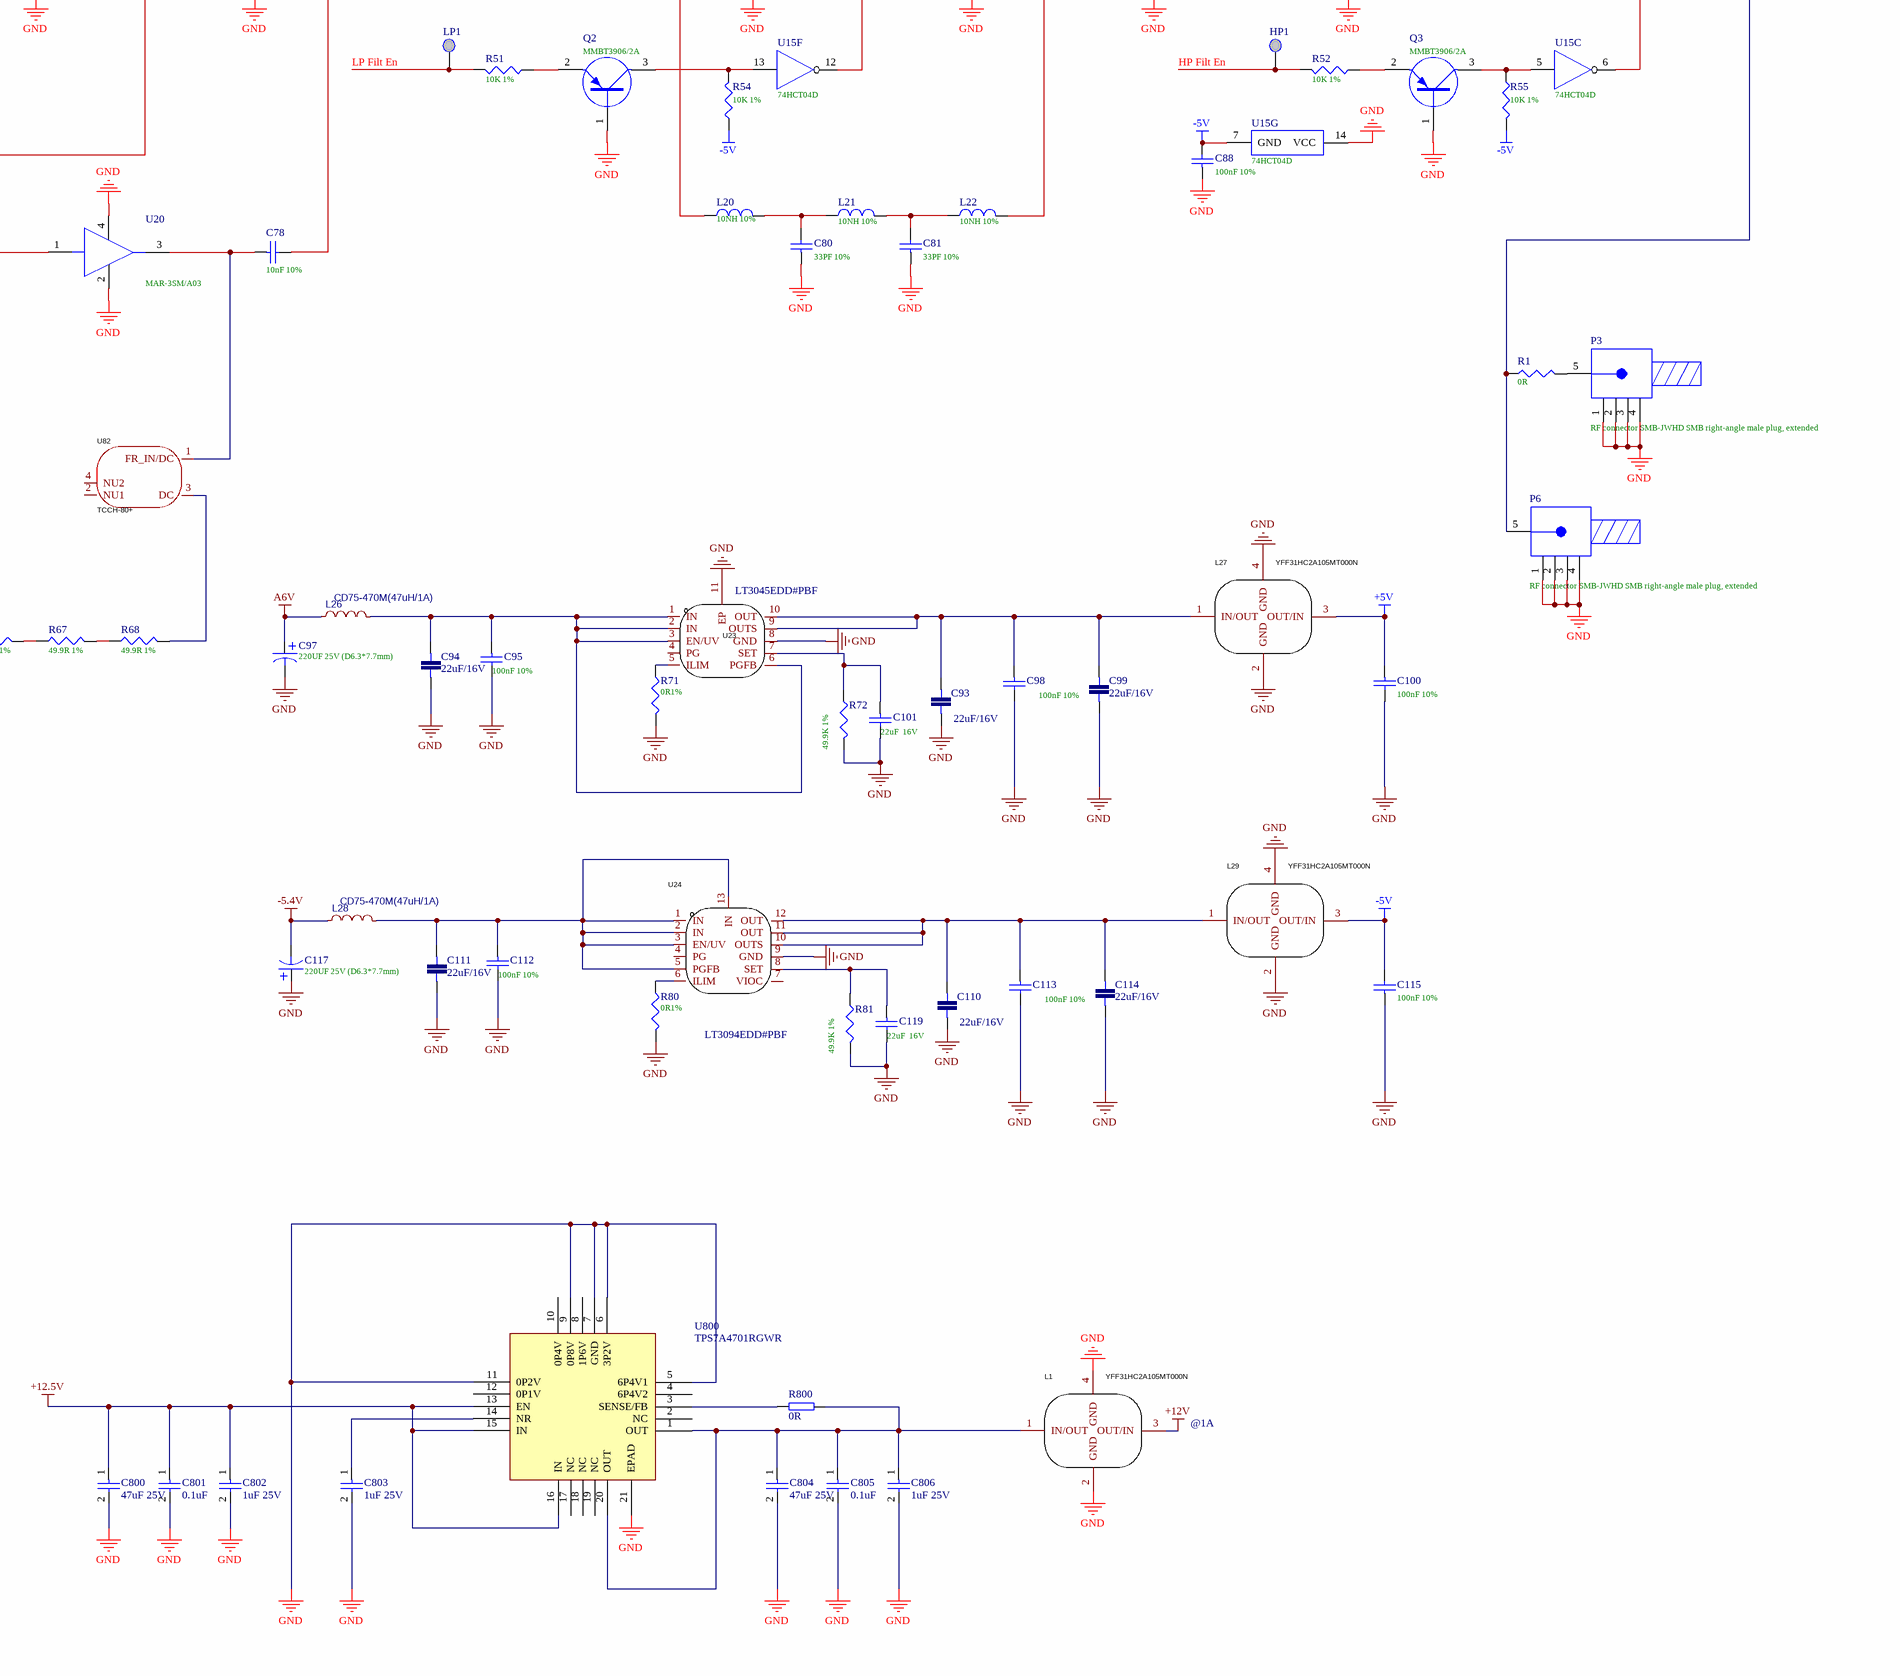
[diagram p0: PCBE109560-12.SchDoc, bottom right]
# Altium project MISC109560-2.PrjPcb (part 2 of 2)

## Sheet PCBE109560-12.SchDoc
size E; SheetNumber: 0; SheetTotal: 0

### Parts
1  (no value)  [DIP-1]
+1  (no value)  [DIP-1]
+2  (no value)  [DIP-1]
C4  20PF 10%  [0805C-2]
C5  330PF 10%  [1812C]
C6  22PF 10%  [1812C-2]
C7  22uF/16V  [0805]
C8  22uF/16V  [0805]
C9  100nF 10%  [0603]
C10  220UF 25V (D6.3*7.7mm)  [CAP-SMD_BD6.3-L6.6-W6.6-FD]
C11  100nF 10%  [0603]
C12  22uF/16V  [0805]
C13  100nF 10%  [0805R]
C14  22uF  16V  [0805]
C15  100nF 10%  [0805R]
C16  47PF 10%  [1812C-2]
C17  100PF 10%  [1812C-2]
C18  20PF 10%  [0805R]
C20  100nF 10%  [0805R]
C21  100nF 10%  [0805R]
C31  100nF 10%  [0805R]
C32  100nF 10%  [0805R]
C34  100nF 10%  [0805R]
C35  100nF 10%  [0805R]
C36  100nF 10%  [0805R]
C37  100nF 10%  [0805R]
C39  100nF 10%  [0805R]
C40  100nF 10%  [0805R]
C41  100nF 10%  [0805R]
C42  100nF 10%  [0805R]
C43  100nF 10%  [0805R]
C44  100nF 10%  [0805R]
C45  100nF 10%  [0805R]
C46  100nF 10%  [0805R]
C47  100nF 10%  [0805R]
C48  100nF 10%  [0805R]
C49  22uF 25V  [CAP-SMD_L6.0-W3.2-R-RD]
C50  100nF 10%  [0805R]
C51  100nF 10%  [0805R]
C52  100nF 10%  [0805R]
C53  3.3NF 10%  [0805R]
C54  100nF 10%  [0805R]
C55  330PF 10%  [0805R]
C56  330PF 10%  [0805R]
C57  100nF 10%  [0805R]
C58  33PF 10%  [0805R]
C59  33PF 10%  [0805R]
C60  100nF 10%  [0805R]
C61  100nF 10%  [0805R]
C62  100nF 10%  [0805R]
C63  100nF 10%  [0805R]
C64  100nF 10%  [0805R]
C65  33PF 10%  [0805R]
C66  33PF 10%  [0805R]
C67  100nF 10%  [0805R]
C68  39PF 10%  [0805R]
C69  100nF 10%  [0805R]
C70  25V 1UF Type A  [0805C-2]
C71  25V 1UF Type A  [0805C-2]
C72  100nF 10%  [0805R]
C73  25V 1UF Type A  [0805C-2]
C74  100nF 10%  [0805R]
C75  100nF 10%  [0805R]
C76  10nF 10%  [0805R]
C77  10nF 10%  [0805R]
C78  10nF 10%  [0805R]
C79  100nF 10%  [0603C]
C80  33PF 10%  [0805R]
C81  33PF 10%  [0805R]
C82  100nF 10%  [0805R]
C83  100nF 10%  [0805R]
C84  100nF 10%  [0805R]
C85  100nF 10%  [0805R]
C86  25V 1UF Type A  [0805C-2]
C87  3pF( ±0.1pF)  [0805R]
C88  100nF 10%  [0805R]
C89  100nF 10%  [0805R]
C90  100nF 10%  [0805R]
C93  22uF/16V  [0805]
C94  22uF/16V  [0805]
C95  100nF 10%  [0603]
C96  100nF 10%  [0805R]
C97  220UF 25V (D6.3*7.7mm)  [CAP-SMD_BD6.3-L6.6-W6.6-FD]
C98  100nF 10%  [0603]
C99  22uF/16V  [0805]
C100  100nF 10%  [0805R]
C101  22uF  16V  [0805]
C102  100nF 10%  [0805R]
C103  100nF 10%  [0805R]
C104  100nF 10%  [0805R]
C105  100nF 10%  [0805R]
C106  100nF 10%  [0805R]
C107  100nF 10%  [0805R]
C109  100nF 10%  [0805R]
C110  22uF/16V  [0805]
C111  22uF/16V  [0805]
C112  100nF 10%  [0603]
C113  100nF 10%  [0603]
C114  22uF/16V  [0805]
C115  100nF 10%  [0805R]
C116  100nF 10%  [0805R]
C117  220UF 25V (D6.3*7.7mm)  [CAP-SMD_BD6.3-L6.6-W6.6-FD]
C118  100nF 10%  [0805R]
C119  22uF  16V  [0805]
C122  100nF 10%  [0805R]
C123  100nF 10%  [0805R]
C124  100nF 10%  [0805R]
C125  100nF 10%  [0805R]
C128  100nF 10%  [0805R]
C129  100nF 10%  [0805R]
C130  100nF 10%  [0805R]
C800  47uF 25V  [1206]
C801  0.1uF  [0402]
C802  1uF 25V  [0402]
C803  1uF 25V  [0402]
C804  47uF 25V  [1206]
C805  0.1uF  [0402]
C806  1uF 25V  [0402]
C809  100nF 10%  [0805R]
C888  100nF 10%  [0805R]
Clk1  (no value)  [DIP-1]
D1  BAV99/A7  [SOT-23]
D2  GF1M-E3/67A/GM  [1808D]
D3  GF1M-E3/67A/GM  [1808D]
D4  GF1M-E3/67A/GM  [1808D]
D5  GF1M-E3/67A/GM  [1808D]
D8  BAV99/A7  [SOT-23-2]
D9  BAV99/A7  [SOT-23-2]
D10  BAV99/A7  [SOT-23-2]
D11  BAV99/A7  [SOT-23-2]
D12  BAV99/A7  [SOT-23-2]
Data1  (no value)  [DIP-1]
HP1  (no value)  [DIP-1]
J1  RF connector  [DIP-P]
J2  RF connector  [DIP-P]
L1  YFF31HC2A105MT000N  [FILTER-SMD_4P-L3.2-W1.6-L_YFF31HC]
L2  15UH 5%  [1005R]
L3  BLM21PG221SN1D(220Ω@100MHz)  [0805R]
L4  YFF31HC2A105MT000N  [FILTER-SMD_4P-L3.2-W1.6-L_YFF31HC]
L5  6.8UH 10%  [0805R]
L8  YFF31HC2A105MT000N  [FILTER-SMD_4P-L3.2-W1.6-L_YFF31HC]
L10  10NH 10%  [0805R]
L11  10NH 10%  [0805R]
L12  10NH 10%  [0805R]
L13  YFF31HC2A105MT000N  [FILTER-SMD_4P-L3.2-W1.6-L_YFF31HC]
L15  4.7UH 5%  [1005L]
L16  1UH 5%  [0805R]
L17  BLM21PG221SN1D(220Ω@100MHz)  [0805R]
L18  BLM21PG221SN1D(220Ω@100MHz  [0805R]
L19  NFM15PC104R1A3D  [FILTER-SMD_0402-3P-L1.0-W0.5-T]
L20  10NH 10%  [0805R]
L21  10NH 10%  [0805R]
L22  10NH 10%  [0805R]
L23  YFF31HC2A105MT000N  [FILTER-SMD_4P-L3.2-W1.6-L_YFF31HC]
L24  YFF31HC2A105MT000N  [FILTER-SMD_4P-L3.2-W1.6-L_YFF31HC]
L25  BLM21PG221SN1D(220Ω@100MHz  [0805R]
L26  CD75-470M(47uH/1A)  [IND-SMD_L7.8-W7.0-A]
L27  YFF31HC2A105MT000N  [FILTER-SMD_4P-L3.2-W1.6-L_YFF31HC]
L28  CD75-470M(47uH/1A)  [IND-SMD_L7.8-W7.0-A]
L29  YFF31HC2A105MT000N  [FILTER-SMD_4P-L3.2-W1.6-L_YFF31HC]
L31  BLM21PG221SN1D(220Ω@100MHz  [0805R]
L32  BLM21PG221SN1D(220Ω@100MHz  [0805R]
L808  NFM15PC104R1A3D  [FILTER-SMD_0402-3P-L1.0-W0.5-T]
L809  NFM15PC104R1A3D  [FILTER-SMD_0402-3P-L1.0-W0.5-T]
L810  NFM15PC104R1A3D  [FILTER-SMD_0402-3P-L1.0-W0.5-T]
L811  NFM15PC104R1A3D  [FILTER-SMD_0402-3P-L1.0-W0.5-T]
L812  NFM15PC104R1A3D  [FILTER-SMD_0402-3P-L1.0-W0.5-T]
L813  NFM15PC104R1A3D  [FILTER-SMD_0402-3P-L1.0-W0.5-T]
LP1  (no value)  [DIP-1]
P1  Header 20X2  [N0.8mm/40Pin-Plug]
P2  Header 4X2  [N0.8mm/8Pin-SOCKET]
P3  RF connector SMB-JWHD SMB right-angle male plug, extended  [DIP-P-2]
P4  Header 20X2  [N0.8mm/40Pin-Plug]
P5  Header 20X2  [N0.8mm/40Pin-Plug]
P6  RF connector SMB-JWHD SMB right-angle male plug, extended  [DIP-P-2]
Q1  MJD31C  [SOT-252-2]
Q2  MMBT3906/2A  [SOT-23]
Q3  MMBT3906/2A  [SOT-23]
Q4  MMBT3906/2A  [SOT-23]
R1  0R  [0805R]
R6  2K 5%  [0603]
R7  NC  [AXIAL-0.51]
R8  3.9K 5% 1/2W  [AXIAL-0.51]
R9  3.9K 5% 1/2W  [AXIAL-0.51]
R10  3.9K 5% 1/2W  [AXIAL-0.51]
R11  3.9K 5% 1/2W  [AXIAL-0.51]
R13  0R1%  [0603]
R14  49.9K 1%  [0603]
R15  4.99K 1%  [0805R]
R16  2K 1%  [0805R]
R17  49.9R 1% 1/4W  [AXIAL-0.4]
R20  100R 1% 1/4W  [AXIAL-0.4]
R23  100R 1% 1/4W  [AXIAL-0.4]
R27  4.87K 1%  [0805R]
R28  4.87K 1%  [0805R]
R29  4.87K 1%  [0805R]
R30  4.87K 1%  [0805R]
R31  4.87K 1%  [0805R]
R32  10K 1%  [0805R]
R33  100K 1%  [0805R]
R34  100K 1%  [0805R]
R35  49.9R 1%  [0805R]
R36  49.9R 1%  [0805R]
R37  49.9R 1%  [0805R]
R38  49.9R 1%  [0805R]
R39  49.9R 1%  [0805R]
R40  49.9R 1% 1/4W  [R-SMD_L3.5-W1.5]
R41  10K 1%  [0805R]
R42  4.87K 1%  [0805R]
R43  4.87K 1%  [0805R]
R44  4.87K 1%  [0805R]
R45  4.87K 1%  [0805R]
R46  169R 1%  [0805R]
R47  169R 1%  [0805R]
R48  169R 1%  [0805R]
R49  49.9R 1%  [0805R]
R50  49.9R 1%  [0805R]
R51  10K 1%  [0805R]
R52  10K 1%  [0805R]
R53  10K 1%  [0805R]
R54  10K 1%  [0805R]
R55  10K 1%  [0805R]
R56  10K 1%  [0805R]
R57  10K 1%  [0805R]
R58  49.9R 1%  [0805R]
R59  4.99K 1%  [0805R]
R60  49.9R 1%  [R-SMD_L3.5-W1.5]
R61  30R 1%  [R-SMD_L3.5-W1.5]
R62  169R 1%  [0805R]
R63  169R 1%  [0805R]
R64  169R 1%  [0805R]
R65  49.9R 1%  [0805R]
R66  49.9R 1%  [0805R]
R67  49.9R 1%  [0805R]
R68  49.9R 1%  [0805R]
R69  120R 1%  [R-SMD_L3.5-W1.5]
R70  169R 1%  [0805R]
R71  0R1%  [0603]
R72  49.9K 1%  [0603]
R73  169R 1%  [0805R]
R74  NC  [0805R]
R75  169R 1%  [0805R]
R77  169R 1%  [0805R]
R80  0R1%  [0603]
R81  49.9K 1%  [0603]
R82  100K 1%  [0805R]
R83  10K 1%  [0805R]
R84  169R 1%  [0805R]
R800  0R  [0402]
RE1  AGQ210A4HZ  [RELAY-SMD_PANASONIC_AGQ2X0AXX]
RE2  AGQ210A4HZ  [RELAY-SMD_PANASONIC_AGQ2X0AXX]
RE3  AGQ210A4HZ  [RELAY-SMD_PANASONIC_AGQ2X0AXX]
RE4  AGQ210A4HZ  [RELAY-SMD_PANASONIC_AGQ2X0AXX]
RE5  AGQ210A4HZ  [RELAY-SMD_PANASONIC_AGQ2X0AXX]
Strobe1  (no value)  [DIP-1]
U4  LT3045EDD#PBF  [DFN-10_L3.0-W3.0-P0.50-BL-EP]
U6  74HCT123D  [SOIC-16_L9.9-W3.9-P1.27-LS6.0-BL]
U8  MAX504CSD+T  [SO-14]
U9  SW-239  [SO-8]
U11  SW-239  [SO-8]
U12  SW-239  [SO-8]
U13  SW-239  [SO-8]
U14  SW-239  [SO-8]
U15  74HCT04D  [SO-14]  (parts A,B,C,D,E,F,G of 7)
U16  AT-250(MAAV-007941)  [SO-8]
U17  MAR-3SM/A03  [LCC4]
U18  MAR-6SM/A06  [LCC4]
U19  MAR-6SM/A06  [LCC4]
U20  MAR-3SM/A03  [LCC4]
U21  MAX4106ESA+T  [SO-8]
U22  MIC4420CM  [SO-8]
U23  LT3045EDD#PBF  [DFN-10_L3.0-W3.0-P0.50-BL-EP]
U24  LT3094EDD#PBF  [WDFN-12_L3.0-W3.0-P0.45-BL-EP]
U25  AT65-0263  [SO-16]
U80  TCCH-80+  [IND-SMD_4P-L3.8-W3.8]
U81  TCCH-80+  [IND-SMD_4P-L3.8-W3.8]
U82  TCCH-80+  [IND-SMD_4P-L3.8-W3.8]
U83  TCCH-80+  [IND-SMD_4P-L3.8-W3.8]
U100  SW-239  [SO-8]
U800  TPS7A4701RGWR  [QFN-20]

### Nets
+5V: C100.1 C888.1 L25.1 L27.3(OUT/IN) L811.3(OUTPUT) L812.3(OUTPUT) U8.3(~{CLR})
+12.5V: +2.1 C106.1 C800.1 C801.1 C802.1 P5.31 P5.32 P5.33 P5.34 P5.35 P5.36 P5.37 P5.38 P5.39 P5.40 U800.13(EN) U800.15(IN) U800.16(IN)
+12V: C122.1 C123.1 C124.2 C125.2 L1.3(OUT/IN) L8.1(IN/OUT) L13.1(IN/OUT) U22.1(VS) U22.8(VS)
-5.4V: +1.1 C107.1 C117.2 L28.2 P5.1 P5.2 P5.3 P5.4 P5.5 P5.6 P5.7 P5.8 P5.9 P5.10
-5V: C88.2 C115.2 L29.3(OUT/IN) L809.1(INPUT) L810.3(OUTPUT) L813.3(OUTPUT) R54.1 R55.2 R57.1 U15.7(GND)
A6V: 1.1 C10.1 C97.1 C103.2 L3.1 L26.2 P5.17 P5.18 P5.19 P5.20 P5.21 P5.22 P5.23 P5.24
GND: C5.1 C6.2 C7.1 C8.1 C9.2 C10.2 C11.2 C12.1 C13.2 C14.2 C15.1 C18.2 C20.1 C21.1 C31.1 C32.1 C34.1 C35.1 C36.2 C37.2 C39.2 C40.2 C42.2 C43.1 C44.2 C45.2 C46.2 C47.1 C48.1 C49.2 C50.2 C57.2 C60.2 C61.1 C62.1 C63.1 C64.1 C65.2 C66.1 C70.1 C71.1 C72.2 C73.1 C74.1 C75.1 C80.1 C81.1 C83.2 C84.2 C85.1 C86.2 C88.1 C89.2 C90.2 C93.1 C94.1 C95.2 C96.2 C97.2 C98.2 C99.1 C100.2 C101.2 C102.2 C103.1 C104.2 C105.1 C106.2 C107.2 C109.2 C110.1 C111.1 C112.2 C113.2 C114.1 C115.1 C117.1 C118.2 C119.2 C122.2 C123.2 C124.1 C125.1 C128.1 C129.1 C130.2 C800.2 C801.2 C802.2 C803.2 C804.2 C805.2 C806.2 C809.2 C888.2 D1.3 D2.2(K) D11.2 D12.1 J1.1 J1.2 J1.3 J1.4 J2.1 J2.2 J2.3 J2.4 L1.2(GND) L1.4(GND) L2.2 L4.2(GND) L4.4(GND) L8.2(GND) L8.4(GND) L13.2(GND) L13.4(GND) L15.2 L16.1 L19.2(GND) L23.2(GND) L23.4(GND) L24.2(GND) L24.4(GND) L27.2(GND) L27.4(GND) L29.2(GND) L29.4(GND) L808.2(GND) L809.2(GND) L810.2(GND) L811.2(GND) L812.2(GND) L813.2(GND) P1.5 P1.6 P1.11 P1.12 P1.17 P1.18 P1.20 P1.23 P1.24 P1.29 P1.30 P1.35 P1.36 P2.1 P2.3 P2.5 P2.7 P3.1 P3.2 P3.3 P3.4 P4.5 P4.6 P4.11 P4.12 P4.17 P4.18 P4.23 P4.24 P4.29 P4.30 P4.35 P4.36 P5.11 P5.12 P5.13 P5.14 P5.15 P5.16 P5.25 P5.26 P5.27 P5.28 P5.29 P5.30 P6.1 P6.2 P6.3 P6.4 Q1.2(E) Q2.1(B) Q3.1(B) Q4.1(B) R13.2 R14.2 R20.2 R32.2 R53.1 R59.1 R61.1 R71.2 R72.2 R74.1 R80.2 R81.2 R82.1 R83.1 RE1.3 RE3.6 RE4.2 U4.8(GND) U4.11(EP) U6.6(2CEXT) U6.8(GND) U6.10(2B) U6.14(1CEXT) U8.7(DGND) U8.8(AGND) U9.2(GND) U9.7(GND) U9.8(GND) U11.2(GND) U11.7(GND) U11.8(GND) U12.2(GND) U12.7(GND) U12.8(GND) U13.2(GND) U13.7(GND) U13.8(GND) U14.2(GND) U14.7(GND) U14.8(GND) U15.14(VCC) U16.2(GND) U16.3(GND) U16.5(GND) U16.6(GND) U16.7(GND) U17.2(GND) U17.4(GND) U18.2(GND) U18.4(GND) U19.2(GND) U19.4(GND) U20.2(GND) U20.4(GND) U22.4(GND) U22.5(GND) U23.8(GND) U23.11(EP) U24.9(GND) U25.2(GND) U25.3(GND) U25.4(GND) U25.5(GND) U25.6(GND) U25.7(GND) U25.16(GND) U100.2(GND) U100.7(GND) U100.8(GND) U800.5(6P4V1) U800.6(3P2V) U800.7(GND) U800.9(0P8V) U800.11(0P2V) U800.21(EPAD)
VCC: C13.1 C15.2 L4.3(OUT/IN) R15.1 R16.2 U6.2(1B) U6.3(1~{R}D) U6.16(VCC)
AK2: C21.2 P1.33 RE1.1
AK3: C20.2 P1.38 RE1.8
AK4: C37.1 P1.37 RE2.1
AK5: C36.1 P1.40 RE2.8
AK6: C31.2 P1.34 RE3.8
AK7: C32.2 P1.32 RE3.1
AK8: C34.2 C40.1 P1.28 RE4.8 RE5.8
AK9: C35.2 C39.1 P1.26 RE4.1 RE5.1
Attn1: P4.34 R70.2
Attn2: P4.32 R73.2
Attn4: P4.28 R75.2
Attn8: P4.26 R77.2
Attn16: P4.22 R84.2
DAC Clk: Clk1.1 P4.14 U8.4(SCLK)
DAC Data: Data1.1 P4.16 U8.2(DIN)
DAC Strobe: P4.10 Strobe1.1 U8.5(~{CS})
DATA_T: P1.39 R15.2 U6.1(1~{A})
HP Filt En: HP1.1 P4.4 R52.2
HT: L5.1 P2.2 P2.4 P2.6 P2.8
IN2: P4.8 R56.1 U22.2(IN)
LP Filt En: LP1.1 P4.2 R51.2
NetC4_1: C4.1 D1.2 L2.1 Q1.1(B) R6.1
NetC4_2: C4.2 R6.2 U6.13(1Q)
NetC5_2: C5.2 L5.2 R7.2
NetC6_1: C6.1 C16.2 C17.2 Q1.3(C) R11.1
NetC7_2: C7.2 C11.1 C12.2 L4.1(IN/OUT) U4.9(OUTS) U4.10(OUT)
NetC8_2: C8.2 C9.1 L3.2 U4.1(IN) U4.2(IN) U4.3(EN/UV) U4.6(PGFB)
NetC14_1: C14.1 R14.1 U4.7(SET)
NetC16_1: C16.1 D5.1(A) D8.2 D9.2 RE2.6
NetC17_1: C17.1 RE2.7
NetC18_1: C18.1 R16.1 U6.15(1REXT/CEXT)
NetC41_1: C41.1 U14.1(RFCOM)
NetC41_2: C41.2 P6.5 R1.1 R32.1
NetC42_1: C42.1 R27.1 U9.5(B)
NetC43_2: C43.2 R28.2 U100.4(A)
NetC44_1: C44.1 R29.1 U11.4(A)
NetC45_1: C45.1 R30.1 U12.5(B)
NetC46_1: C46.1 R31.1 U13.5(B) U14.4(A)
NetC47_2: C47.2 R35.1 U16.4(A)
NetC48_2: C48.2 L8.3(OUT/IN) R36.1
NetC49_1: C49.1 C50.1 U8.1(BIPOFF) U8.9(REFIN) U8.10(REFOUT)
NetC51_1: C51.1 U17.1(RF_IN)
NetC51_2: C51.2 U16.8(RF2)
NetC52_1: C52.1 L10.2
NetC52_2: C52.2 U17.3(RF_OUT) U81.1(FR_IN/DC)
NetC53_1: C53.1 C54.1 L15.1
NetC53_2: C53.2 U12.1(RFCOM)
NetC54_2: C54.2 U13.1(RFCOM)
NetC55_1: C55.1 U13.3(RF1)
NetC55_2: C55.2 C56.1 L16.2
NetC56_2: C56.2 U14.6(RF2)
NetC57_1: C57.1 R41.1 U13.4(A) U14.5(B)
NetC58_1: C58.1 C65.1
NetC58_2: C58.2 L10.1 L11.1
NetC59_1: C59.1 L11.2 L12.1
NetC59_2: C59.2 C66.2
NetC60_1: C60.1 R42.1 U9.4(A)
NetC61_2: C61.2 R43.2 U100.5(B)
NetC62_2: C62.2 R44.1 U11.5(B)
NetC63_2: C63.2 R45.1 U12.4(A)
NetC64_2: C64.2 L13.3(OUT/IN) R46.2
NetC67_1: C67.1 U18.1(RF_IN)
NetC67_2: C67.2 U25.1(RF)
NetC68_1: C68.1 C69.2 R49.2 R50.2
NetC68_2: C68.2 R49.1 R50.1 U18.3(RF_OUT) U80.1(FR_IN/DC)
NetC69_1: C69.1 R53.2 U16.1(RF1)
NetC70_2: C70.2 C74.2 L18.1 L19.1(INPUT)
NetC71_2: C71.2 C75.2 L19.3(OUTPUT) U21.4(VEE)
NetC72_1: C72.1 C73.2 L17.2 L18.2
NetC76_1: C76.1 U9.3(RF1)
NetC76_2: C76.2 U19.1(RF_IN)
NetC77_1: C77.1 U19.3(RF_OUT) U83.1(FR_IN/DC)
NetC77_2: C77.2 U20.1(RF_IN)
NetC78_1: C78.1 U20.3(RF_OUT) U82.1(FR_IN/DC)
NetC78_2: C78.2 U100.6(RF2)
NetC79_1: C79.1 D10.3 R40.2
NetC79_2: C79.2 R58.2 R59.2
NetC80_2: C80.2 L20.2 L21.2
NetC81_2: C81.2 L21.1 L22.1
NetC82_1: C82.1 R60.2
NetC82_2: C82.2 C116.1 R74.2 R82.2
NetC83_1: C83.1 C86.1 L808.1(INPUT) U21.7(VCC)
NetC84_1: C84.1 L23.3(OUT/IN) R62.2
NetC85_2: C85.2 L24.3(OUT/IN) R65.1
NetC87_1: C87.1 R60.1 R69.1 U21.6(OUT)
NetC87_2: C87.2 R61.2 R69.2 U21.2(IN-)
NetC89_1: C89.1 L813.1(INPUT) U8.11(VSS)
NetC90_1: C90.1 L32.2 L811.1(INPUT)
NetC93_2: C93.2 C98.1 C99.2 L27.1(IN/OUT) U23.9(OUTS) U23.10(OUT)
NetC94_2: C94.2 C95.1 L26.1 U23.1(IN) U23.2(IN) U23.3(EN/UV) U23.6(PGFB)
NetC96_1: C96.1 R70.1 U25.15(C1)
NetC101_1: C101.1 R72.1 U23.7(SET)
NetC102_1: C102.1 R73.1 U25.14(C2)
NetC104_1: C104.1 L812.1(INPUT) U8.13(VDD)
NetC105_2: C105.2 L31.1 L810.1(INPUT)
NetC109_1: C109.1 R75.1 U25.13(C4)
NetC110_2: C110.2 C113.1 C114.2 L29.1(IN/OUT) U24.10(OUTS) U24.11(OUT) U24.12(OUT)
NetC111_2: C111.2 C112.1 L28.1 U24.1(IN) U24.2(IN) U24.3(EN/UV) U24.5(PGFB) U24.13(IN)
NetC116_2: C116.2 R83.2 U25.8(RF)
NetC118_1: C118.1 R77.1 U25.12(C8)
NetC119_1: C119.1 R81.1 U24.8(SET)
NetC128_2: C128.2 L31.2 U25.11(VEE)
NetC129_2: C129.2 L32.1 U25.10(VCC)
NetC130_1: C130.1 R84.1 U25.9(C16)
NetC803_1: C803.1 U800.14(NR)
NetC804_1: C804.1 C805.1 C806.1 L1.1(IN/OUT) R800.1 U800.1(OUT) U800.20(OUT)
NetC809_1: C809.1 L25.2 L808.3(OUTPUT)
NetD2_1: D2.1(A) D3.2(K)
NetD3_1: D3.1(A) D4.2(K)
NetD4_1: D4.1(A) D5.2(K)
NetD8_1: D8.1 D9.1 J1.5 R17.1 R20.1 R23.1 RE4.4
NetD10_1: D10.1 D12.2
NetD10_2: D10.2 D11.1
NetJ2_5: J2.5 RE5.4
NetL12_2: L12.2 U9.1(RFCOM)
NetL17_1: L17.1 L809.3(OUTPUT)
NetL20_1: L20.1 U11.6(RF2)
NetL22_2: L22.2 U12.3(RF1)
NetL23_1: L23.1(IN/OUT) L24.1(IN/OUT) U22.6(OUT) U22.7(OUT)
NetP3_5: P3.5 R1.2
NetQ2_2: Q2.2(E) R51.1
NetQ2_3: Q2.3(C) R54.2 U15.13(6A)
NetQ3_2: Q3.2(E) R52.1
NetQ3_3: Q3.3(C) R55.1 U15.5(3A)
NetQ4_2: Q4.2(E) R56.2
NetQ4_3: Q4.3(C) R57.2 U15.1(1A)
NetR7_1: R7.1 R8.1
NetR8_2: R8.2 R9.2
NetR9_1: R9.1 R10.1
NetR10_2: R10.2 R11.2
NetR13_1: R13.1 U4.5(ILIM)
NetR17_2: R17.2 RE1.2
NetR23_2: R23.2 RE3.7
NetR27_2: R27.2 R28.1 U15.4(2Y)
NetR29_2: R29.2 R30.2 U15.10(5Y)
NetR31_2: R31.2 U15.8(4Y)
NetR33_1: R33.1 R34.1 U8.14(RFB)
NetR33_2: R33.2 R34.2 R35.2 U8.12(VOUT)
NetR36_2: R36.2 R37.1
NetR37_2: R37.2 R38.2
NetR38_1: R38.1 R39.1
NetR39_2: R39.2 U81.3(DC)
NetR40_1: R40.1 RE5.3
NetR41_2: R41.2 U15.6(3Y) U15.9(4A)
NetR42_2: R42.2 R43.1 U15.2(1Y) U15.3(2A)
NetR44_2: R44.2 R45.2 U15.11(5A) U15.12(6Y)
NetR46_1: R46.1 R47.2
NetR47_1: R47.1 R48.1
NetR48_2: R48.2 U80.3(DC)
NetR58_1: R58.1 U21.3(IN+)
NetR62_1: R62.1 R63.1
NetR63_2: R63.2 R64.2
NetR64_1: R64.1 U83.3(DC)
NetR65_2: R65.2 R66.2
NetR66_1: R66.1 R67.1
NetR67_2: R67.2 R68.1
NetR68_2: R68.2 U82.3(DC)
NetR71_1: R71.1 U23.5(ILIM)
NetR80_1: R80.1 U24.6(ILIM)
NetR800_2: R800.2 U800.3(SENSE/FB)
NetRE4_3: RE4.3 RE5.2
NetU9_6: U9.6(RF2) U100.3(RF1)
NetU11_1: U11.1(RFCOM) U100.1(RFCOM)
NetU11_3: U11.3(RF1) U12.6(RF2)
NetU13_6: U13.6(RF2) U14.3(RF1)

Not connected (* = marked no-connect by the designer): D1 1*; D8 3; D9 3; D11 3; D12 3; P1 1 2 3 4 7 8 9 10 13 14 15 16 19 21 22 25 27 31; P4 1 3 7 9 13 15 19 20 21 25 27 31 33 37 38 39 40; RE1 4 5 6 7; RE2 2 3 4 5; RE3 2 3 4 5; RE4 5 6 7; RE5 5 6 7; U4 4(PG); U6 4(1~{Q}) 5(2Q) 7(2REXT/CEXT) 9(2~{A}) 11(2~{R}D) 12(2~{Q}); U8 6(DOUT); U22 3(NC); U23 4(PG); U24 4(PG) 7(VIOC); U80 2(NU1) 4(NU2); U81 2(NU1) 4(NU2); U82 2(NU1) 4(NU2); U83 2(NU1) 4(NU2); U800 2(NC) 4(6P4V2) 8(1P6V) 10(0P4V) 12(0P1V) 17(NC) 18(NC) 19(NC)

### Notes on the sheet
- (near P1) Transmit interface
- 500V high-voltage interface
- Receive interface
- @1A

### Library data of the parts
1 +1 +2 Clk1 Data1 HP1 LP1 Strobe1 = TP
C4-C6 C9 C11 C13-C18 C20 C21 C31 C32 C34-C37 C39-C48 C50-C69 C72-C85 C87-C90 C95 C96 C98 C100-C107 C109 C112 C113 C115 C116 C118 C119 C122-C125 C128-C130 C800-C806 C809 C888 = CAP: Capacitor
C7 C8 C12 C93 C94 C99 C110 C111 C114 = C1206
C10 C97 C117 = CAPACITOR_1: Capacitor
C49 = TAJC226K025RNJ: Manufacturer: Kyocera AVX; Add into BOM: yes; Tolerance: ±10%; Equivalent Series Resistance(ESR): 1.4Ω@100kHz; Symbol: TAJC226K025RNJ; Device: TAJC226K025RNJ; LCSC Part Name: 22uF ±10% 25V; Supplier Part: C7214; Manufacturer Part: TAJC226K025RNJ; Supplier Footprint: CASE-C-6032; JLCPCB Part Class: Extended Part; Datasheet: https://atta.szlcsc.com/upload/public/pdf/source/20160107/1457707750344.pdf; Supplier: LCSC; Convert to PCB: yes; Value: 22uF; Rated Voltage: 25V; Operating Temperature: -55℃~+125℃
C70 C71 C86 = CAPACITOR POL: Capacitor
D1 D8-D12 = BAV99
D2-D5 = DIODE
J1 J2 = SMA-KWE: BOM_Supplier: *; BOM_Supplier Part: *; BOM_Manufacturer: *; BOM_Manufacturer Part: *; BOM_JLCPCB Part Class: *; spicePre: *; spiceSymbolName: *; Contributor: *
L1 L4 L8 L13 L23 L24 L27 L29 = YFF31HC2A105MT000N: Manufacturer: TDK; Add into BOM: yes; Nominal Capacitance: 1uF; CapacitanceTolerance: ±20%; DC Rated Voltage: 100V; Rated Current: 6A; DC Resistance: 5mΩ; Name: YFF31HC2A105MT000N; Symbol: YFF31HC2A105MT000N; Device: YFF31HC2A105MT000N; LCSC Part Name: 1uF(105) ±20% 100V; Supplier Part: C113216; Manufacturer Part: YFF31HC2A105MT000N; Supplier Footprint: SMD-4P,1.6x3.2mm; JLCPCB Part Class: Extended Part; Datasheet: https://atta.szlcsc.com/upload/public/pdf/source/20180326/C113216_F6F81E50B9805DA3D7C436129903DEBD.pdf; Supplier: LCSC; Convert to PCB: yes; Operating Temperature: -55℃~+125℃
L2 L3 L5 L10-L12 L15-L18 L20-L22 L25 L31 L32 = INDUCTOR
L19 L808-L813 = NFM15PC104R1A3D: Manufacturer: muRata(村田); Add into BOM: yes; Nominal Capacitance: 100nF; CapacitanceTolerance: ±20%; DC Rated Voltage: 10V; Rated Current: 2A; DC Resistance: 30mΩ; Symbol: NFM15PC104R1A3D; Device: NFM15PC104R1A3D; LCSC Part Name: 0.1uF ±20% 10V; Supplier Part: C2650905; Manufacturer Part: NFM15PC104R1A3D; Supplier Footprint: 0402; JLCPCB Part Class: Extended Part; Datasheet: https://atta.szlcsc.com/upload/public/pdf/source/20210611/05FD8D968916F804F398094FB2B4AAFE.pdf; Supplier: LCSC; Convert to PCB: yes; Operating Temperature: -55℃~+105℃; Comment_1: NFM15PC104R1A3D
L26 L28 = 4.7uH/5a: BOM_Manufacturer: COILMX; BOM_Manufacturer Part: MS0630-4R7M; nameAlias: Inductance; Contributor: LCSC; BOM_Supplier: LCSC; BOM_Supplier Part: C380177; spicePre: L; spiceSymbolName: MS0630-4R7M
P1 P4 P5 = Header 20X2: Header, 20-Pin, Dual row; LatestRevisionDate: 17-Jul-2002; LatestRevisionNote: Re-released for DXP Platform.; Publisher: Altium Limited
P2 = Header 4X2: Header, 4-Pin, Dual row; LatestRevisionDate: 17-Jul-2002; LatestRevisionNote: Re-released for DXP Platform.; Publisher: Altium Limited
P3 P6 = JA1
Q1 = NPN: NPN Transistor
Q2-Q4 = PNP: PNP Transistor
R1 R6-R11 R13-R17 R20 R23 R27-R75 R77 R80-R84 = RES1
R800 = RES
RE1-RE5 = AGQ210A4HZ: Manufacturer: PANASONIC(松下); Add into BOM: yes; Coil Voltage: 4.5V; Contact Form: Two changeover sets: 2C (DPDT changeover); Maximum Switching Voltage: 125V@AC; 110V@DC; Coil Type: Single coil; Maximum Switching Current: 2A; Operate Time: 4ms; Symbol: AGQ210A4HZ; Device: AGQ210A4HZ; LCSC Part Name: AGQ210A4HZ; Supplier Part: C2153577; Manufacturer Part: AGQ210A4HZ; Supplier Footprint: SMD,7.2x10.6mm; JLCPCB Part Class: Extended Part; Datasheet: https://atta.szlcsc.com/upload/public/pdf/source/20210727/C2858037_82AE1FE69E1888D41D6E9B5D42950540.pdf; Supplier: LCSC; Convert to PCB: yes; Pin Number: -; Contact Rating: -; Contact Material: AgPd + gold plating; Coil Rated Power: -; Coil Resistance: -; Release Time: 4ms; Contact Resistance: -; Operating Temperature: -40℃~+85℃; Comment_1: AGQ210A4HZ
U4 U23 = LT3045EDD#PBF: Symbol: LT3045EDD#PBF_C666574; Add into BOM: yes; Maximum Input Voltage: 20V; Output Voltage: 0V~15V; MAX Output Current: 500mA; Dropout Voltage: 450mV@(500mA); standby current: 20uA; Number of Outputs: 1; Device: LT3045EDD#PBF; LCSC Part Name: LT3045EDD#PBF; Supplier Part: C666574; Manufacturer Part: LT3045EDD#PBF; Supplier Footprint: DFN-10-EP(3x3); JLCPCB Part Class: Extended Part; Datasheet: https://atta.szlcsc.com/upload/public/pdf/source/20200416/C514420_E440C492D6C74EAE6AB301243586F696.pdf; Supplier: LCSC; Convert to PCB: yes
U15 = 74HC04
U16 = AT-250
U17 U20 = MAR-3SM
U18 U19 = MAR-6SM
U21 = MAX4107ESA: Manufacturer: *; Manufacturer Part: *; Supplier Part: *; Supplier: *; link: *; spicePre: *; spiceSymbolName: *; Package Display: *; Contributor: *
U24 = LT3094EDD#PBF: Add into BOM: yes; Symbol: LT3094EDD#PBF; Device: LT3094EDD#PBF; LCSC Part Name: LT3094EDD#PBF; Supplier Part: C670492; Manufacturer Part: LT3094EDD#PBF; Supplier Footprint: WDFN-12-EP(3x3); JLCPCB Part Class: Extended Part; Datasheet: https://atta.szlcsc.com/upload/public/pdf/source/20200318/C498217_A5485280C797CF3891C55BEBE66C21D4.pdf; Supplier: LCSC; Convert to PCB: yes; Output Type: -
U80-U83 = TCCH-80+: Manufacturer: Mini-Circuits; Add into BOM: yes; Value: 4uH; Rated Current: 200mA; DC Resistance (DCR): 100mΩ; Symbol: TCCH-80+; Device: TCCH-80+; LCSC Part Name: 4uH; Supplier Part: C3223029; Manufacturer Part: TCCH-80+; Supplier Footprint: SMD-4P,3.8x3.8mm; JLCPCB Part Class: Extended Part; Datasheet: https://atta.szlcsc.com/upload/public/pdf/source/20240402/75EC49D4FFFA61CBEC009CC2CCA83C83.pdf; Supplier: LCSC; Convert to PCB: yes; Tolerance: -; Saturation Current (Isat): -; Type: -; Ratings: -
U800 = TPS7A4701RGWR(QFN20): Name: *; Symbol: *; Device: *; LCSC Part Name: *; Supplier Part: *; Manufacturer: *; Manufacturer Part: *; Supplier Footprint: *; JLCPCB Part Class: *; Datasheet: *; Supplier: *; Add into BOM: *; Convert to PCB: *; Output Type: *; Output Polarity: *; Number of Outputs: *